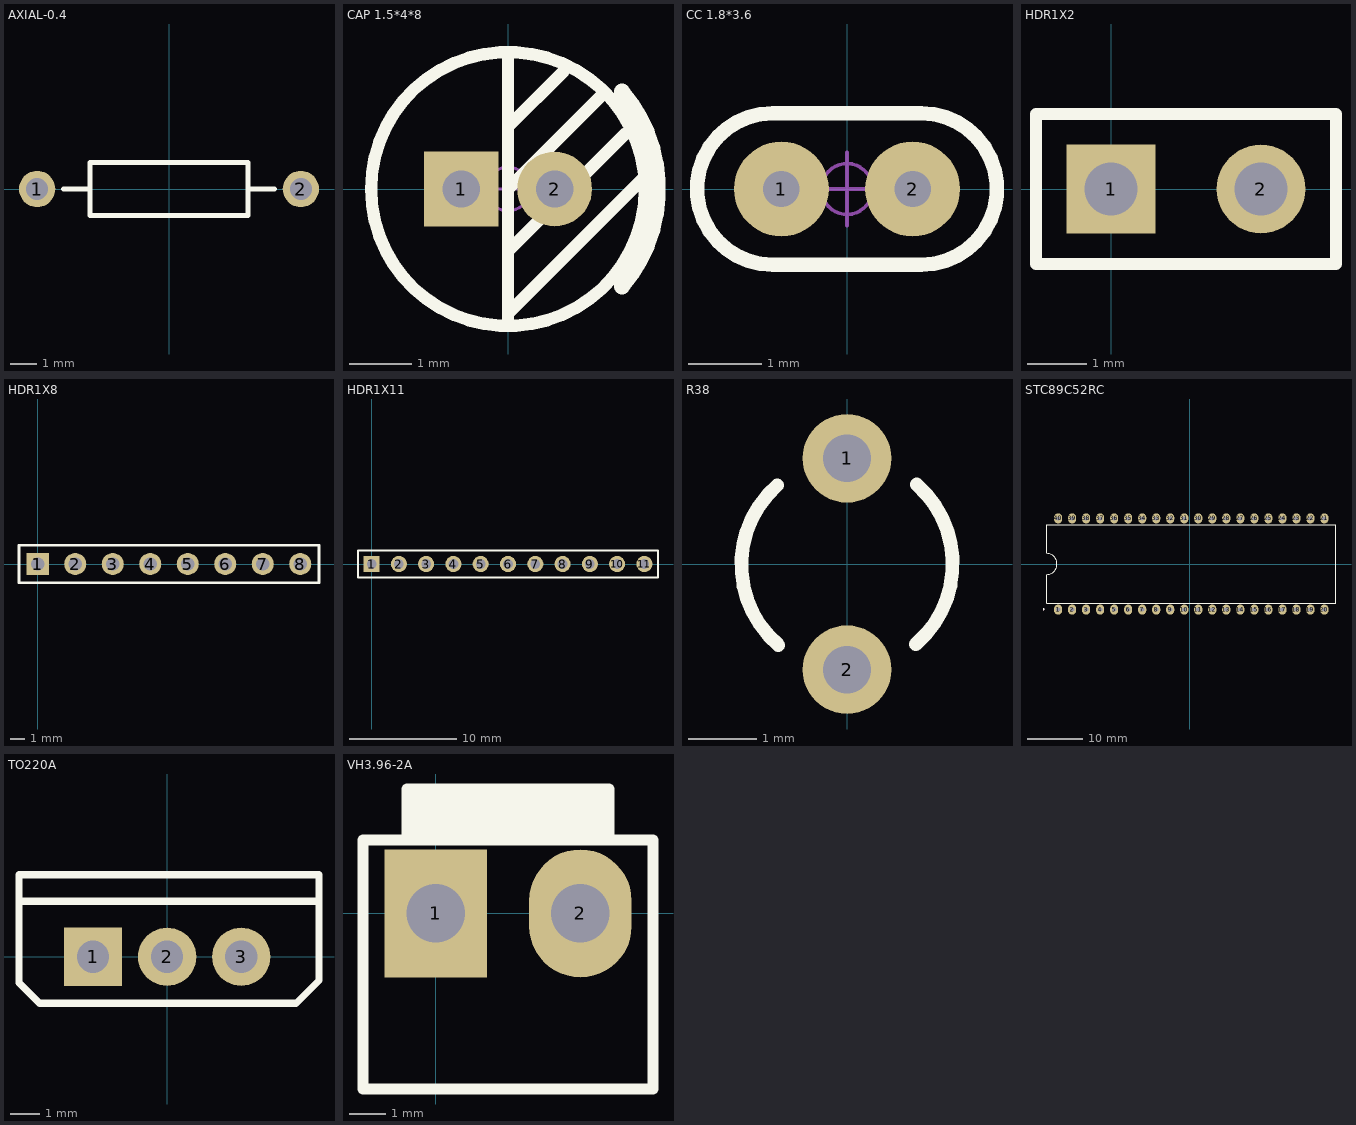
[diagram p0: the footprints below, top view; thin cyan lines are the x and y axes]
# Altium footprint library MISC80679.PcbLib: 10 footprints
Each footprint in its own frame and in the unit in brackets; x right, y up, seen from the top. Pads: shape width x height; smd on the part's side, far side on the other; paste and mask are expansions set on the pad; w line width, h text height; cw(c..) or ccw(c..) is an arc to the next point about the centre after c.

## AXIAL-0.4 [mm] "Axial Device, Thru-Hole; 2 Leads; 0.4 in Pin Spacing"
height 2.032
pads (2):
  round 1.4 hole 0.85: 1(-5.08,0) 2(5.08,0)
Top Overlay:
  lines w0.2: -4.064,0 -3.048,0 ; 3.048,0 4.064,0 ; -3.048,-1.016 3.048,-1.016 3.048,1.016 -3.048,1.016 -3.048,-1.016

## CAP 1.5*4*8 [mm] "pin pitch 1.5mm, diameter 4mm, height 8mm"
height 4.58
pads (2):
  rect 1.2x1.2 hole 0.6: 1(-0.75,0)
  round 1.2 hole 0.6: 2(0.75,0)
Top Overlay:
  circle w0.2: c0,0 r2.2
  lines w0.2: 0,-2.159 0,-2 ; 0,-1 1.897,0.897 ; 0,0 1.524,1.524 ; 0,1 0.897,1.897 ; 0,2.159 0,-2 ; 2.207,0.206 0,-2
  lines w0.254: 1.83,-1.568 ccw(c0,0) 1.83,1.568
Mechanical 15:
  circle w0.05: c0,0 r0.35
  lines w0.05: -0.5,0 0.5,0 ; 0,-0.5 0,0.5
3D body "CAP 1.5X4X8.STEP": height 8.04, standoff -3.46, extent -2,-1.999 2.02,1.999

## CC 1.8*3.6 [mm] "pin pitch 1.8mm, diameter 3.6mm"
height 4.58
pads (2):
  round 1.3 hole 0.5: 1(-0.9,0) 2(0.9,0)
Top Overlay:
  lines w0.2: -1.016,-1.041 cw(c-1.016,0) -1.016,1.041 1.016,1.041 cw(c1.016,0) 1.016,-1.041 -1.016,-1.041
Mechanical 15:
  circle w0.05: c0,0 r0.35
  lines w0.05: -0.5,0 0.5,0 ; 0,-0.5 0,0.5
3D body "CC 1.8X3.6.STEP": height 3.6, standoff -3.5, extent -1.8,-0.798 1.8,0.796

## HDR1X2 [mm] "Connector; Header; 2 Position"
height 4.58
pads (2):
  rect 1.5x1.5 hole 0.9: 1(0,0)
  round 1.5 hole 0.9: 2(2.54,0)
Top Overlay:
  lines w0.2: -1.27,-1.27 -1.27,1.27 3.81,1.27 3.81,-1.27 -1.27,-1.27

## HDR1X8 [mm] "Connector; Header; 8 Position"
height 4.58
pads (8):
  rect 1.5x1.5 hole 0.9: 1(0,0)
  round 1.5 hole 0.9: 2(2.54,0) 3(5.08,0) 4(7.62,0) 5(10.16,0) 6(12.7,0) 7(15.24,0) 8(17.78,0)
Top Overlay:
  lines w0.2: -1.27,-1.27 19.05,-1.27 19.05,1.27 -1.27,1.27 -1.27,-1.27

## HDR1X11 [mm] "Connector; Header; 11 Position"
height 4.58
pads (11):
  rect 1.5x1.5 hole 0.9: 1(0,0)
  round 1.5 hole 0.9: 2(2.54,0) 3(5.08,0) 4(7.62,0) 5(10.16,0) 6(12.7,0) 7(15.24,0) 8(17.78,0) 9(20.32,0) 10(22.86,0) 11(25.4,0)
Top Overlay:
  lines w0.2: -1.27,-1.27 -1.27,1.27 0.635,1.27 26.67,1.27 26.67,-1.27 -1.27,-1.27

## R38 [mm] "Crystal, Thru-Hole; 2 Leads; Body 3.1 x 8.2 mm (Dia.xH)"
height 8.2
pads (2):
  round 1.3 hole 0.7: 1(0,1.55) 2(0,-1.55)
Top Overlay:
  lines w0.2: -1.022,1.155 ccw(c0,-0.01) -1.006,-1.189 ; 1.006,-1.179 ccw(c0,0) 1.022,1.165

## STC89C52RC [mm]
height 4.58
pads (40):
  oval 1.467x1.833 hole 0.8 paste+0 mask+0.051: 1(-23.868,-8.255) 2(-21.328,-8.255) 3(-18.788,-8.255) 4(-16.248,-8.255) 5(-13.708,-8.255) 6(-11.168,-8.255) 7(-8.628,-8.255) 8(-6.088,-8.255) 9(-3.548,-8.255) 10(-1.008,-8.255) 11(1.532,-8.255) 12(4.072,-8.255) 13(6.612,-8.255) 14(9.152,-8.255) 15(11.692,-8.255) 16(14.232,-8.255) 17(16.772,-8.255) 18(19.312,-8.255) 19(21.852,-8.255) 20(24.392,-8.255) 21(24.392,8.255) 22(21.852,8.255) 23(19.312,8.255) 24(16.772,8.255) 25(14.232,8.255) 26(11.692,8.255) 27(9.152,8.255) 28(6.612,8.255) 29(4.072,8.255) 30(1.532,8.255) 31(-1.008,8.255) 32(-3.548,8.255) 33(-6.088,8.255) 34(-8.628,8.255) 35(-11.168,8.255) 36(-13.708,8.255) 37(-16.248,8.255) 38(-18.788,8.255) 39(-21.328,8.255) 40(-23.868,8.255)
Top Overlay:
  circle w0.15: c-26.502,-8.222 r0.075
  lines w0.152: -25.976,-7.11 -25.976,-1.905 ccw(c-25.976,0) -25.976,1.905 -25.976,7.11 26.501,7.11 26.501,-7.11 -25.976,-7.11
Mechanical 15:
  circle w0.15: c-26.502,-8.222 r0.075

## TO220A [mm] "220, 3-pin transistor"
height 4.58
pads (3):
  rect 2x2 hole 1.1: 1(-2.54,0)
  round 2 hole 1.1: 2(0,0) 3(2.54,0)
Top Overlay:
  lines w0.254: -4.928,1.905 5.131,1.905 ; -5.08,-0.889 -5.08,2.819 5.207,2.819 5.207,-0.813 4.42,-1.6 -4.369,-1.6 -5.08,-0.889
3D body "4.STEP": height 18.5, standoff -4, extent -5.08,-1.453 5.22,2.977

## VH3.96-2A [mm]
height 4.58
pads (2):
  rect 2.8x3.5 hole 1.6: 1(0,0)
  oval 2.8x3.5 hole 1.6: 2(3.96,0)
Top Overlay:
  lines w0.3: -0.78,2 -0.78,3.4 4.74,3.4 4.74,2 ; -0.78,2.286 4.74,2.286 ; -0.78,2.413 4.74,2.413 ; -0.78,2.667 4.74,2.667 ; -0.78,2.921 4.74,2.921 ; -0.78,3.175 4.74,3.175 ; -1.98,-4.8 -1.98,2 5.94,2 5.94,-4.8 -1.98,-4.8
3D body "VH3.96-2A.STEP": height 14.6, standoff -3.6, extent -1.98,-4.8 5.94,3.6